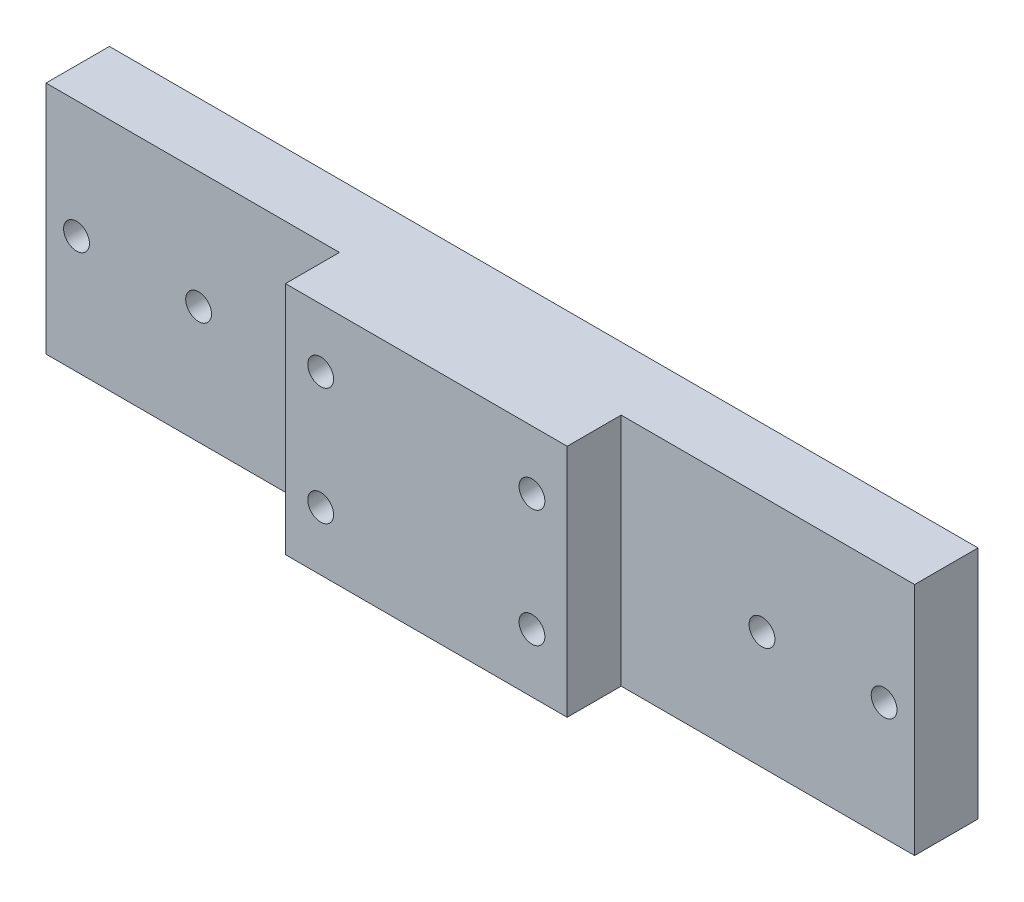
SolidWorks part; units mm, degrees
ref_plane "Front Plane" through (0, 0, 0) normal (0, 0, 1) x (1, 0, 0)
ref_plane "Top Plane" through (0, 0, 0) normal (0, 1, 0) x (1, 0, 0)
ref_plane "Right Plane" through (0, 0, 0) normal (1, 0, 0) x (0, 0, -1)
sketch "Sketch1" plane through (0, 0, 0) normal (0, 0, 1) x (1, 0, 0)
  line L0 (-92.5, 25) -> (92.5, -25) construction
  line L1 (-92.5, 25) -> (92.5, 25)
  line L2 (-92.5, 25) -> (-92.5, -25)
  line L3 (-92.5, -25) -> (92.5, -25)
  line L4 (92.5, 25) -> (92.5, -25)
  line L5 (92.5, -25) -> (92.0958, -24.1916) construction
  dimension "D1" = 185
  dimension "D2" = 50
extrude "Boss-Extrude1" add sketch "Sketch1" along normal blind 25
sketch "Sketch2" plane through (0, 0, 25) normal (0, 0, 1) x (1, 0, 0)
  line L0 (-92.5, -25) -> (92.5, -25) construction
  line L1 (-92.5, 25) -> (-30, 25)
  line L2 (-92.5, 25) -> (-92.5, -25)
  line L3 (-92.5, -25) -> (-30, -25)
  line L4 (-30, 25) -> (-30, -25)
  line L6 (92.5, 25) -> (30, 25)
  line L7 (92.5, 25) -> (92.5, -25)
  line L8 (92.5, -25) -> (30, -25)
  line L9 (30, 25) -> (30, -25)
  dimension "D1" = 60
extrude "Cut-Extrude1" cut sketch "Sketch2" against normal blind 11.5
hole_wizard "M5 socket head cap screw counterbore1" positions "Sketch4" profile "Sketch3" counterbore size "M5" standard "Gb" end condition through all
sketch "Sketch4" plane through (0, 0, 0) normal (0, 0, -1) x (-1, 0, 0)
  line L1 (-92.5, -25) -> (-92.5, 25) construction
  line L2 (92.5, 25) -> (92.5, -25) construction
  line L3 (0, 0) -> (-60, 0) construction
  point P0 (-86, 0)
  point P2 (-60, 0)
  point P4 (60, 0)
  point P6 (86, 0)
  dimension "D1" = 26
  dimension "D2" = 6.5
  dimension "D3" = 6.5
  dimension "D4" = 26
sketch "Sketch3" plane through (86, 0, 0) normal (1, 0, 0) x (0, 1, 0)
  line L0 (0, 0) -> (0, 25)
  line L1 (0, 25) -> (2.75, 25)
  line L3 (2.75, 25) -> (2.75, 5.7)
  line L4 (2.75, 5.7) -> (5, 5.7)
  line L5 (5, 5.7) -> (5, 0)
  line L7 (5, 0) -> (0, 0)
  line L11 (0, -6.35) -> (0, 107.95) construction
  dimension "貫穿孔直徑" = 5.5
  dimension "貫穿孔深度" = 25
  dimension "柱孔直徑" = 10
  dimension "柱孔深度" = 5.7
hole_wizard "M5 socket head cap screw counterbore2" positions "Sketch6" profile "Sketch5" counterbore size "M5" standard "Gb" end condition through all
sketch "Sketch6" plane through (0, 0, 0) normal (0, 0, -1) x (-1, 0, 0)
  line L0 (0, 0) -> (0, 25) construction
  line L1 (-92.5, 25) -> (92.5, 25) construction
  line L3 (0, 0) -> (36.3051, 0) construction
  point P0 (-22.5, 12.5)
  point P2 (-22.5, -12.5)
  point P4 (22.5, 12.5)
  point P6 (22.5, -12.5)
  dimension "D1" = 45
  dimension "D2" = 25
sketch "Sketch5" plane through (22.5, 12.5, 0) normal (1, 0, 0) x (0, 1, 0)
  line L0 (0, 0) -> (0, 25)
  line L1 (0, 25) -> (2.75, 25)
  line L3 (2.75, 25) -> (2.75, 5.7)
  line L4 (2.75, 5.7) -> (5, 5.7)
  line L5 (5, 5.7) -> (5, 0)
  line L7 (5, 0) -> (0, 0)
  line L11 (0, -6.35) -> (0, 107.95) construction
  dimension "貫穿孔直徑" = 5.5
  dimension "貫穿孔深度" = 25
  dimension "柱孔直徑" = 10
  dimension "柱孔深度" = 5.7
